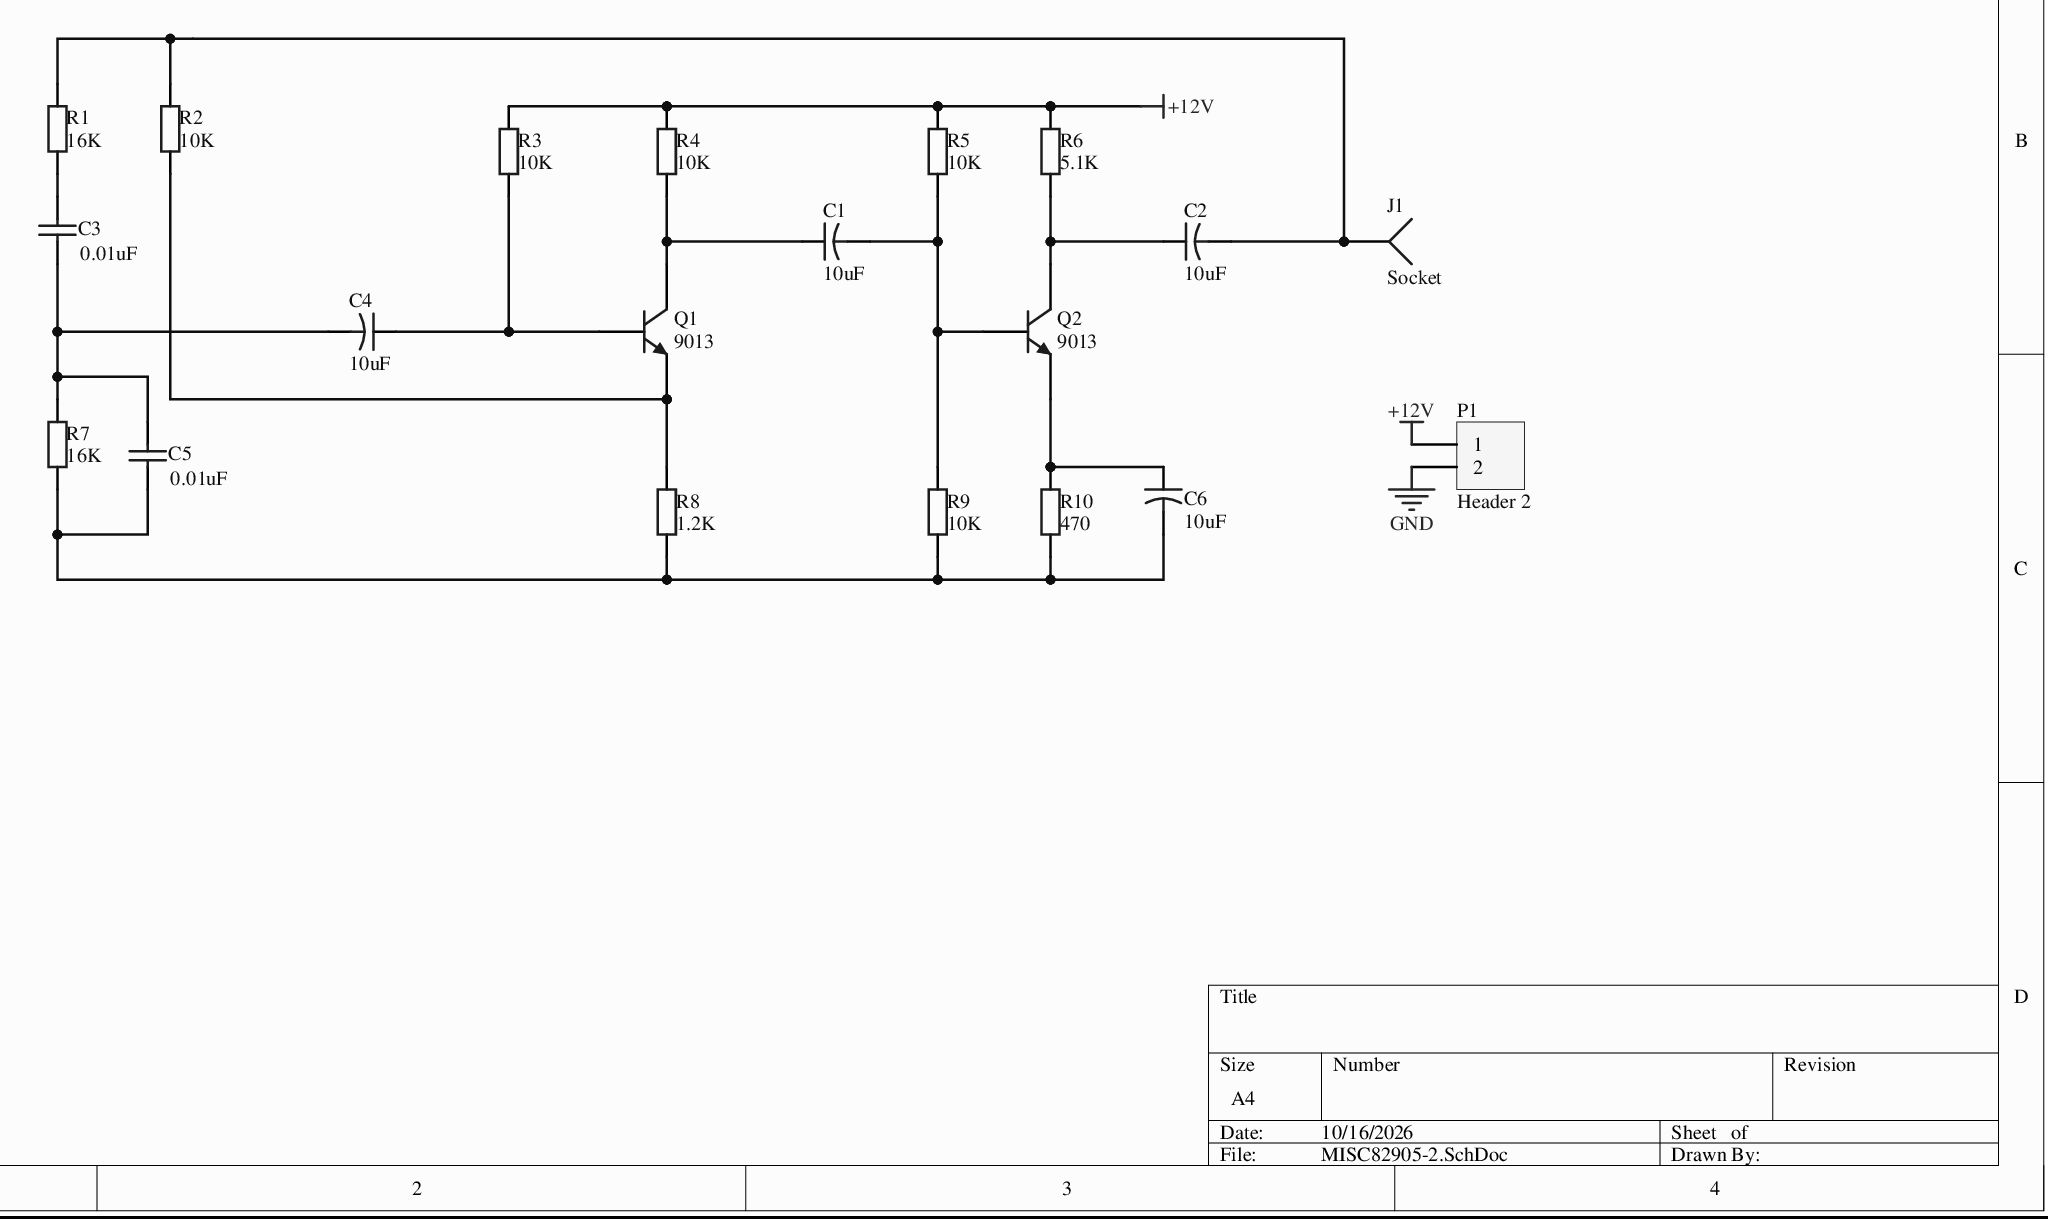
[diagram p0: MISC82905-2.SchDoc]
# Altium project MISC82905-5.PrjPcb
1 sheet, 20 parts. Net scope: global (net labels, ports and power ports of the same name join across sheets).
Board file: MISC82905.PcbDoc

## Sheet MISC82905-2.SchDoc
size A4

### Parts
C1  10uF  [CAPR5-4X5]
C2  10uF  [CAPR5-4X5]
C3  0.01uF  [RAD-0.3]
C4  10uF  [CAPR5-4X5]
C5  0.01uF  [RAD-0.3]
C6  10uF  [CAPR5-4X5]
J1  Socket  [PIN1]
P1  Header 2  [HDR1X2]
Q1  9013  [TO-92A]
Q2  9013  [TO-92A]
R1  16K  [AXIAL-0.4]
R2  10K  [AXIAL-0.4]
R3  10K  [AXIAL-0.4]
R4  10K  [AXIAL-0.4]
R5  10K  [AXIAL-0.4]
R6  5.1K  [AXIAL-0.4]
R7  16K  [AXIAL-0.4]
R8  1.2K  [AXIAL-0.4]
R9  10K  [AXIAL-0.4]
R10  470  [AXIAL-0.4]

### Nets
+12V: P1.1 R3.2 R4.2 R5.2 R6.2
GND: P1.2
NetC1_1: C1.1 Q1.3(C) R4.1
NetC1_2: C1.2 Q2.2(B) R5.1 R9.2
NetC2_1: C2.1 Q2.3(C) R6.1
NetC2_2: C2.2 J1.1 R1.2 R2.2
NetC3_1: C3.1 C4.2 C5.2 R7.2
NetC3_2: C3.2 R1.1
NetC4_1: C4.1 Q1.2(B) R3.1
NetC5_1: C5.1 C6.2 R7.1 R8.1 R9.1 R10.1
NetC6_1: C6.1 Q2.1(E) R10.2
NetQ1_1: Q1.1(E) R2.1 R8.2

### Library data of the parts
C1 C2 C4 C6 = Cap2: Capacitor; Value: 100pF; Published: 23-Sep-2002; PackageReference: CAPR5-4X5; PackageDescription: Capacitor; 2 Leads; Publisher: Altium Limited
C3 C5 = Cap: Capacitor; Value: 100pF; Published: 8-Jun-2000; LatestRevisionDate: 17-Jul-2002; LatestRevisionNote: Re-released for DXP Platform.; PackageReference: RAD-0.3; PackageDescription: Radial Cap, Thru-Hole; 2 Leads; 0.3 in Pin Spacing; Publisher: Altium Limited
P1 = Header 2: Header, 2-Pin; LatestRevisionDate: 17-Jul-2002; LatestRevisionNote: Re-released for DXP Platform.; Publisher: Altium Limited
Q1 Q2 = 2N3904: NPN General Purpose Amplifier; Published: 8-Jun-2000; LatestRevisionDate: 15-Jan-2003; LatestRevisionNote: PCB Footprint 'BCY-W3/D4.7' replaced; DatasheetVersion: 1997; PackageVersion: Sep-1998; PackageReference: TO-92A; PackageDescription: TO, Flat Index; 3 In-Line, Axial Leads; Body Dia. 4.5mm; Leads 0.51 x 0.48 mm (max); ComponentLink1Description: Manufacturer Link; ComponentLink2Description: Datasheet; ComponentLink2URL: http://www.fairchildsemi.com/ds/2N%2F2N3904.pdf; Publisher: Altium Limited
R1-R10 = Res2: Resistor; Value: 1K; Published: 8-Jun-2000; LatestRevisionDate: 17-Jul-2002; LatestRevisionNote: Re-released for DXP Platform.; PackageReference: AXIAL-0.4; PackageDescription: Axial Device, Thru-Hole; 2 Leads; 0.4 in Pin Spacing; Publisher: Altium Limited
J1 = Socket: LatestRevisionDate: 17-Jul-2002; LatestRevisionNote: Re-released for DXP Platform.; Publisher: Altium Limited